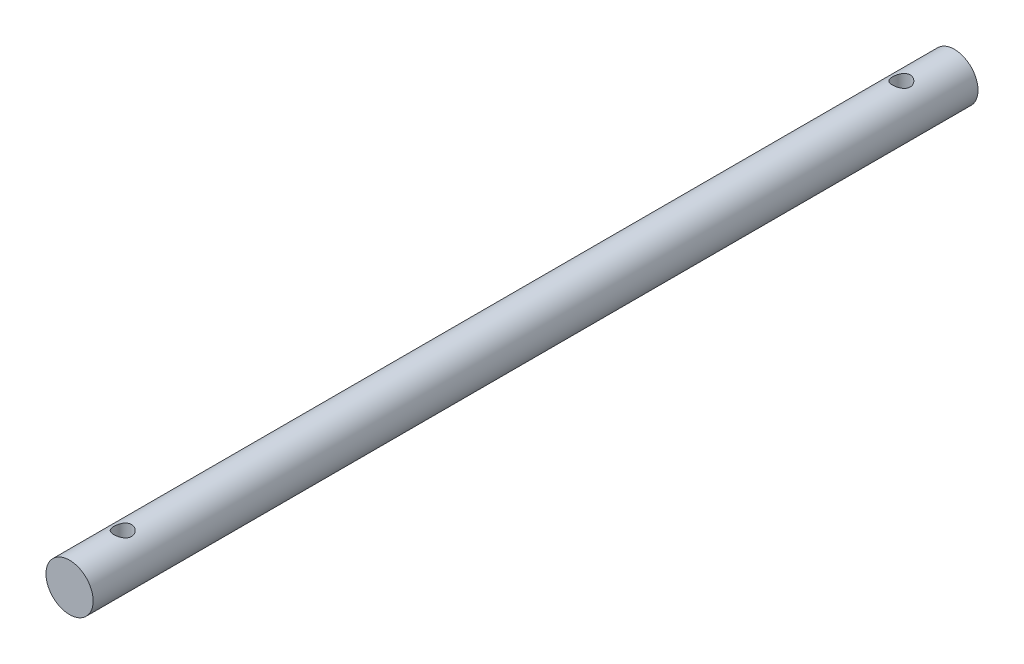
SolidWorks part; units mm, degrees
ref_plane "Front Plane" through (0, 0, 0) normal (0, 0, 1) x (1, 0, 0)
ref_plane "Top Plane" through (0, 0, 0) normal (0, 1, 0) x (1, 0, 0)
ref_plane "Right Plane" through (0, 0, 0) normal (1, 0, 0) x (0, 0, -1)
sketch "Sketch1" plane through (0, 0, 0) normal (0, 0, 1) x (1, 0, 0)
  circle A0 centre (0, 0) radius 4
  dimension "D1" = 8
extrude "Boss-Extrude1" add sketch "Sketch1" along normal mid plane 150
sketch "Sketch3" plane through (0, 0, 0) normal (0, 1, 0) x (1, 0, 0)
  line L0 (4, 75) -> (-4, 75) construction
  line L1 (-4, -75) -> (4, -75) construction
  circle A0 centre (0, 66) radius 1.5
  circle A1 centre (0, -66) radius 1.5
  dimension "D1" = 3
  dimension "D3" = 3
  dimension "D2" = 9
  dimension "D4" = 9
extrude "Cut-Extrude1" cut sketch "Sketch3" against normal mid plane 10
